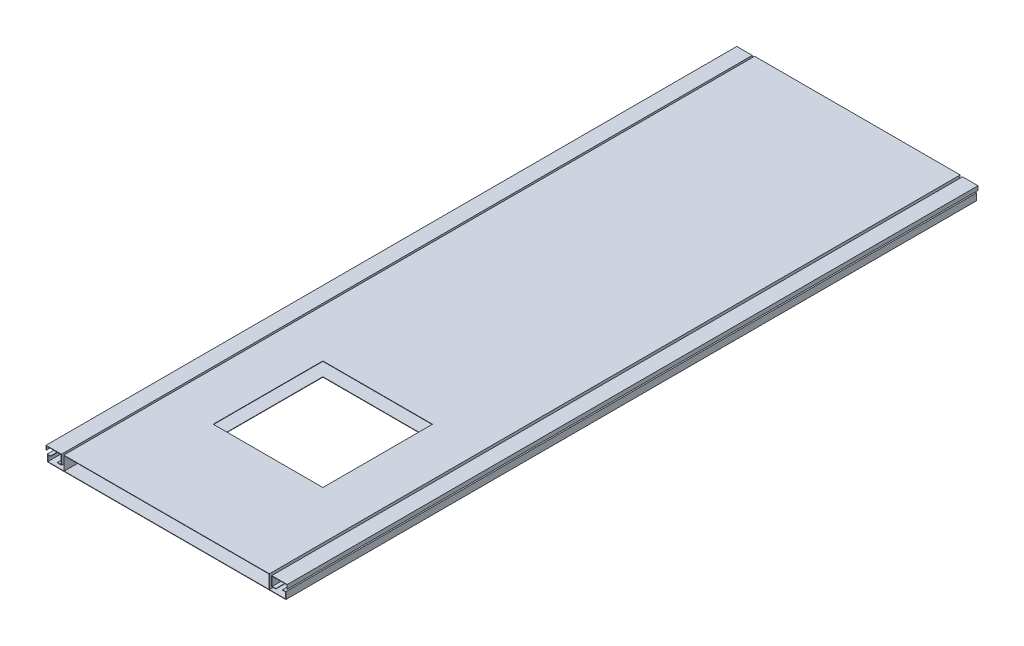
from build123d import *

# Parameters (mm, degrees)
BOSS_EXTRUDE1_DEPTH   = 2520
BOSS_EXTRUDE1_2_DEPTH = 2520
BOSS_EXTRUDE1_3_DEPTH = 2520
BOSS_EXTRUDE2_DEPTH   = 2520
SKETCH2_W             = 400
SKETCH2_H             = 400
CUT_EXTRUDE1_DEPTH    = 2669.084940552


with BuildPart() as part:
    # Sketch 1_3 → Boss-Extrude1 (new body)
    with BuildSketch(Plane.XY):
        Polygon((820, 48.5), (873.5, 48.5), (873.5, 35), (875, 35), (875, 50), (818.5, 50), (818.5, 15), (833.5, 15), (833.5, 16.5), (820, 16.5), align=None)
    extrude(amount=BOSS_EXTRUDE1_DEPTH)


with BuildPart() as body_2:
    # Sketch 1_3 → Boss-Extrude1 2 (new body)
    with BuildSketch(Plane.XY):
        Polygon((-3.5, 48.5), (-3.5, 35), (-5, 35), (-5, 50), (51.5, 50), (51.5, 15), (36.5, 15), (36.5, 16.5), (50, 16.5), (50, 48.5), align=None)
    extrude(amount=BOSS_EXTRUDE1_2_DEPTH)


with BuildPart() as body_3:
    # Sketch 1_3 → Boss-Extrude1 3 (new body)
    with BuildSketch(Plane.XY):
        Polygon((61.5, 1.5), (61.5, 50), (808.5, 50), (808.5, 1.5), (810, 1.5), (810, 51.5), (60, 51.5), (60, 1.5), align=None)
    extrude(amount=BOSS_EXTRUDE1_3_DEPTH)


with BuildPart() as body_4:
    # Sketch 1_3 2 → Boss-Extrude2 (new body)
    with BuildSketch(Plane.XY):
        Polygon((1.5, 23.5), (12, 23.5), (12, 25), (0, 25), (0, 0), (870, 0), (870, 25), (858, 25), (858, 23.5), (868.5, 23.5), (868.5, 1.5), (810, 1.5), (808.5, 1.5), (61.5, 1.5), (60, 1.5), (1.5, 1.5), align=None)
    extrude(amount=BOSS_EXTRUDE2_DEPTH)


with BuildPart() as cut_extrude1_tool:
    # Sketch2 → Cut-Extrude1 (new, through all)
    with BuildSketch(Plane.XZ):
        with Locations((435, 1950)):
            Rectangle(SKETCH2_W, SKETCH2_H)
    extrude(amount=-CUT_EXTRUDE1_DEPTH)


with BuildPart() as body_3_1:
    add(body_3.part)

    # Cut-Extrude1: cut by cut_extrude1_tool
    add(cut_extrude1_tool.part, mode=Mode.SUBTRACT)


with BuildPart() as body_4_1:
    add(body_4.part)

    # Cut-Extrude1: cut by cut_extrude1_tool
    add(cut_extrude1_tool.part, mode=Mode.SUBTRACT)


solid = Compound([part.part, body_2.part, body_3_1.part, body_4_1.part])
